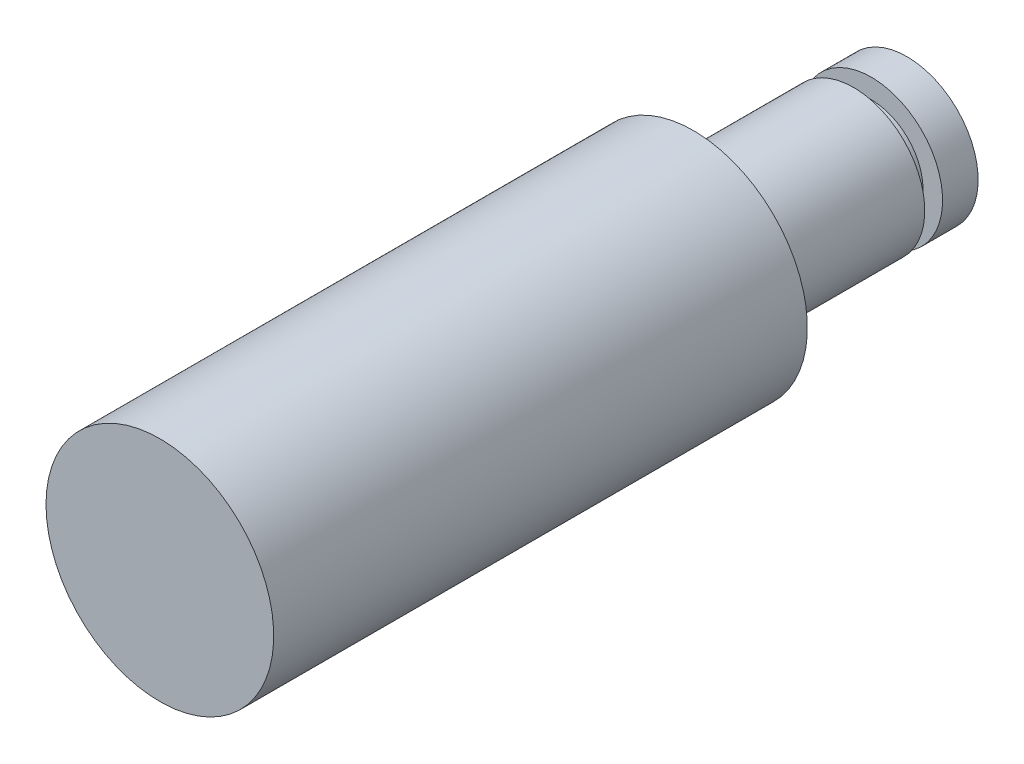
SolidWorks part; units mm, degrees
ref_plane "前视基准面" through (0, 0, 0) normal (0, 0, 1) x (1, 0, 0)
ref_plane "上视基准面" through (0, 0, 0) normal (0, 1, 0) x (1, 0, 0)
ref_plane "右视基准面" through (0, 0, 0) normal (1, 0, 0) x (0, 0, -1)
sketch "草图1" plane through (0, 0, 0) normal (0, 1, 0) x (1, 0, 0)
  line L0 (0, 0) -> (0, -16604.0523) construction
  line L1 (0, 0) -> (-4, 0)
  line L2 (-4, 0) -> (-4, -2)
  line L8 (-4, -2) -> (-2.9, -2)
  line L9 (-2.9, -2) -> (-2.9, -3)
  line L10 (-2.9, -3) -> (-4, -3)
  line L11 (-4, -3) -> (-4, -12)
  line L13 (-4, -12) -> (-6.4, -12)
  line L14 (-6.4, -12) -> (-6.4, -42)
  line L15 (-6.4, -42) -> (0, -42)
  line L16 (0, -42) -> (0, 0)
  point P15 (-3.45, -2)
  dimension "D1" = 12.8
  dimension "D2" = 1
  dimension "D3" = 9
  dimension "D4" = 1.1
  dimension "D5" = 8
  dimension "D6" = 30
  dimension "D7" = 2
revolve "旋转1" add sketch "草图1" angle 360 about L0
